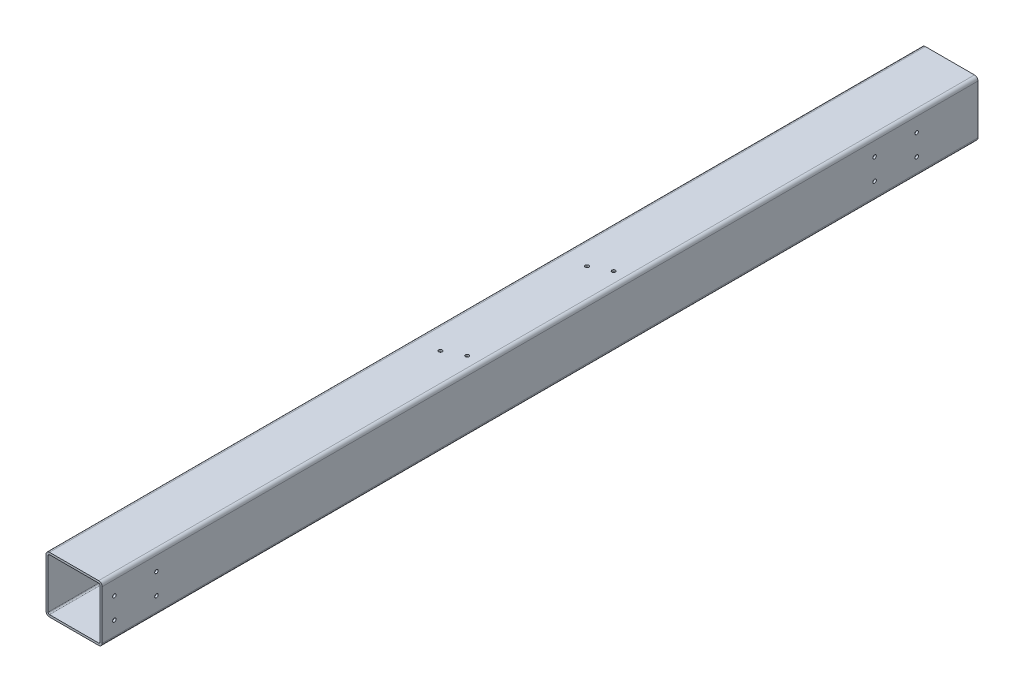
SolidWorks part; units mm, degrees
material "1023 碳钢板 (SS)"
ref_plane "前视基准面" through (0, 0, 0) normal (0, 0, 1) x (1, 0, 0)
ref_plane "上视基准面" through (0, 0, 0) normal (0, 1, 0) x (1, 0, 0)
ref_plane "右视基准面" through (0, 0, 0) normal (1, 0, 0) x (0, 0, -1)
sketch "草图1" plane through (0, 0, 0) normal (0, 0, 1) x (1, 0, 0)
  line L1 (40, 40) -> (-40, 40)
  line L2 (40, 40) -> (40, -40)
  line L3 (40, -40) -> (-40, -40)
  line L4 (-40, 40) -> (-40, -40)
  line L5 (40, 40) -> (-40, -40) construction
  line L6 (40, -40) -> (-40, 40) construction
  point P0 (0, 0)
  dimension "D1" = 80
  dimension "D2" = 80
extrude "凸台-拉伸1" add sketch "草图1" along normal blind 1249
fillet "圆角1" radius 5 4 edges at (-40, -40, 624.5) (40, -40, 624.5) (-40, 40, 624.5) (40, 40, 624.5)
shell "抽壳1" thickness 3
sketch "草图2" plane through (40, 0, 0) normal (1, 0, 0) x (0, 0, -1)
  line L0 (0, -40) -> (-1249, -40) construction
  line L1 (-1231.5, -15) -> (-1171.5, -15) construction
  line L2 (-1231.5, -15) -> (-1231.5, 15) construction
  line L3 (-1231.5, 15) -> (-1171.5, 15) construction
  line L4 (-1171.5, -15) -> (-1171.5, 15) construction
  line L5 (-1231.5, -15) -> (-1171.5, 15) construction
  line L6 (-1231.5, 15) -> (-1171.5, -15) construction
  line L7 (-1249, -35) -> (-1249, 35) construction
  line L9 (-147.5, 15) -> (-87.5, 15) construction
  line L10 (-147.5, 15) -> (-147.5, -15) construction
  line L11 (-147.5, -15) -> (-87.5, -15) construction
  line L12 (-87.5, 15) -> (-87.5, -15) construction
  line L13 (-147.5, 15) -> (-87.5, -15) construction
  line L14 (-147.5, -15) -> (-87.5, 15) construction
  circle A0 centre (-1231.5, 15) radius 2
  circle A1 centre (-1171.5, 15) radius 2
  circle A2 centre (-1171.5, -15) radius 2
  circle A3 centre (-1231.5, -15) radius 2
  circle A4 centre (-147.5, 15) radius 2
  circle A5 centre (-87.5, 15) radius 2
  circle A6 centre (-87.5, -15) radius 2
  circle A7 centre (-147.5, -15) radius 2
  point P0 (-1201.5, 0)
  point P13 (-117.5, 0)
  dimension "D5" = 4
  dimension "D10" = 4
  dimension "D1" = 60
  dimension "D2" = 30
  dimension "D3" = 40
  dimension "D4" = 17.5
  dimension "D6" = 60
  dimension "D7" = 87.5
  dimension "D8" = 30
  dimension "D9" = 40
hole_wizard "M6 螺纹孔1" positions "草图3" profile "草图4" tap size "M6" standard "ISO"
sketch "草图3" plane through (40, 0, 0) normal (1, 0, 0) x (0, 0, -1)
  point P0 (-147.5, 15)
  point P3 (-87.5, 15)
  point P6 (-87.5, -15)
  point P9 (-147.5, -15)
  point P12 (-1171.5, 15)
  point P15 (-1171.5, -15)
  point P18 (-1231.5, -15)
  point P21 (-1231.5, 15)
sketch "草图4" plane through (40, 15, 147.5) normal (0, 1, 0) x (0, 0, -1)
  line L0 (0, 0) -> (0, 16.5022)
  line L1 (0, 16.5022) -> (2.5, 15)
  line L2 (2.5, 15) -> (2.5, 0)
  line L5 (2.5, 0) -> (0, 0)
  line L10 (0, 16.5022) -> (-2.5, 15) construction
  line L11 (0, -6.35) -> (0, 107.95) construction
  dimension "螺纹孔钻头直径" = 5
  dimension "螺纹孔钻头深度" = 15
  dimension "导头角度" = 118
cosmetic thread "孔螺蚊线1"
cosmetic thread "孔螺蚊线2"
cosmetic thread "孔螺蚊线3"
cosmetic thread "孔螺蚊线4"
cosmetic thread "孔螺蚊线5"
cosmetic thread "孔螺蚊线6"
cosmetic thread "孔螺蚊线7"
cosmetic thread "孔螺蚊线8"
sketch "草图5" plane through (0, -40, 0) normal (0, -1, 0) x (1, 0, 0)
  line L0 (40, 1249) -> (40, 0) construction
  line L1 (-35, 0) -> (35, 0) construction
  line L2 (-35, 1249) -> (35, 1249) construction
  circle A0 centre (20, 749.5) radius 2
  circle A1 centre (-5, 736.5) radius 2
  circle A2 centre (20, 540.5) radius 2
  circle A3 centre (-5, 527.5) radius 2
  dimension "D6" = 4
  dimension "D1" = 13
  dimension "D2" = 13
  dimension "D3" = 25
  dimension "D4" = 20
  dimension "D5" = 527.5
  dimension "D7" = 499.5
hole_wizard "M6 螺纹孔2" positions "草图6" profile "草图7" tap size "M6" standard "ISO"
sketch "草图6" plane through (0, -40, 0) normal (0, -1, 0) x (-1, 0, 0)
  point P0 (-20, -749.5)
  point P3 (5, -736.5)
  point P6 (-20, -540.5)
  point P9 (5, -527.5)
sketch "草图7" plane through (20, -40, 749.5) normal (1, 0, 0) x (0, 0, -1)
  line L0 (0, 0) -> (0, 16.5022)
  line L1 (0, 16.5022) -> (2.5, 15)
  line L2 (2.5, 15) -> (2.5, 0)
  line L5 (2.5, 0) -> (0, 0)
  line L10 (0, 16.5022) -> (-2.5, 15) construction
  line L11 (0, -6.35) -> (0, 107.95) construction
  dimension "螺纹孔钻头直径" = 5
  dimension "螺纹孔钻头深度" = 15
  dimension "导头角度" = 118
cosmetic thread "孔螺蚊线9"
cosmetic thread "孔螺蚊线10"
cosmetic thread "孔螺蚊线11"
cosmetic thread "孔螺蚊线12"
sketch "草图8" plane through (0, 40, 0) normal (0, 1, 0) x (1, 0, 0)
  line L1 (-35, -1249) -> (35, -1249) construction
  line L2 (40, -1249) -> (40, 0) construction
  line L3 (35, 0) -> (-35, 0) construction
  circle A0 centre (20, -499.5) radius 2
  circle A1 centre (-5, -512.5) radius 2
  circle A2 centre (20, -708.5) radius 2
  circle A3 centre (-5, -721.5) radius 2
  dimension "D7" = 4
  dimension "D3" = 499.5
  dimension "D1" = 13
  dimension "D2" = 13
  dimension "D4" = 527.5
  dimension "D5" = 20
  dimension "D6" = 25
hole_wizard "M6 螺纹孔3" positions "草图9" profile "草图10" tap size "M6" standard "ISO"
sketch "草图9" plane through (0, 40, 0) normal (0, 1, 0) x (1, 0, 0)
  point P0 (-5, -721.5)
  point P3 (20, -708.5)
  point P6 (20, -499.5)
  point P9 (-5, -512.5)
sketch "草图10" plane through (-5, 40, 721.5) normal (1, 0, 0) x (0, 0, 1)
  line L0 (0, 0) -> (0, 16.5022)
  line L1 (0, 16.5022) -> (2.5, 15)
  line L2 (2.5, 15) -> (2.5, 0)
  line L5 (2.5, 0) -> (0, 0)
  line L10 (0, 16.5022) -> (-2.5, 15) construction
  line L11 (0, -6.35) -> (0, 107.95) construction
  dimension "螺纹孔钻头直径" = 5
  dimension "螺纹孔钻头深度" = 15
  dimension "导头角度" = 118
cosmetic thread "孔螺蚊线13"
cosmetic thread "孔螺蚊线14"
cosmetic thread "孔螺蚊线15"
cosmetic thread "孔螺蚊线16"
